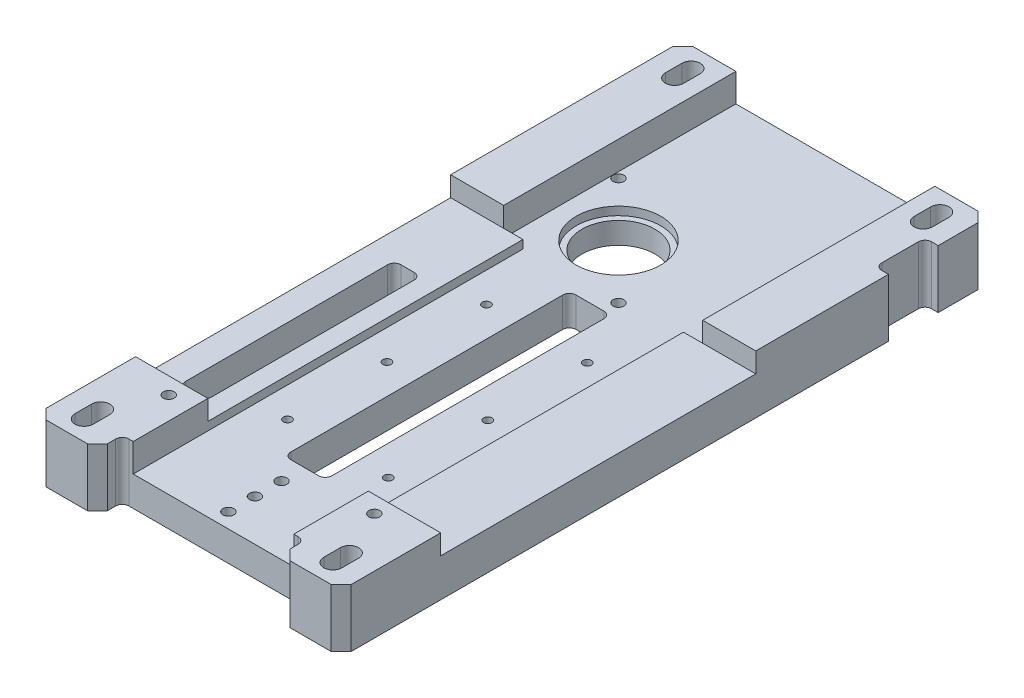
from build123d import *

# Parameters (mm, degrees)
SKETCH1_W               = 92
SKETCH1_H               = 230
BOSS_EXTRUDE1_DEPTH     = 17.5
SKETCH3_W               = 92
SKETCH3_H               = 20
CUT_EXTRUDE2_DEPTH      = 57
SKETCH7_W               = 92
SKETCH7_H               = 35
CUT_EXTRUDE5_DEPTH      = 70
SKETCH6_W               = 48.4
SKETCH6_H               = 175
CUT_EXTRUDE4_DEPTH      = 8.5
M3_TAPPED_HOLE1_D       = 2.5
SKETCH4_W               = 12.4
SKETCH4_H               = 86
CUT_EXTRUDE3_DEPTH      = 29
CHAMFER1_SIZE           = 3
FILLET1_R               = 2
SKETCH2_R               = 11
CUT_EXTRUDE1_DEPTH      = 10
BOSS_EXTRUDE2_DEPTH     = 20
CUT_EXTRUDE9_DEPTH      = 144.69150984
CHAMFER2_SIZE           = 3
SKETCH22_W              = 8
SKETCH22_H              = 65
CUT_EXTRUDE10_DEPTH     = 144.69150984
FILLET2_R               = 2
SKETCH12_R              = 12.75
CUT_EXTRUDE7_DEPTH      = 2.5
SKETCH23_W              = 92
SKETCH23_H              = 95
CUT_EXTRUDE11_DEPTH     = 6
M2_5_TAPPED_HOLE1_D     = 2.05
M2_5_TAPPED_HOLE1_DEPTH = 6.35
M2_5_TAPPED_HOLE1_TIP   = 0.615882135
M4_TAPPED_HOLE4_D       = 3.3
M4_TAPPED_HOLE4_DEPTH   = 10.1
M4_TAPPED_HOLE4_TIP     = 0.991420021
SKETCH16_R              = 1
CUT_EXTRUDE8_DEPTH      = 10
SKETCH30_W              = 4
SKETCH30_H              = 15
CUT_EXTRUDE12_DEPTH     = 144.69150984
M4_TAPPED_HOLE2_D       = 3.3
FILLET3_R               = 2
LPATTERN1_COUNT         = 3
LPATTERN1_PITCH         = 8
SKETCH31_W              = 55
SKETCH31_H              = 15
CUT_EXTRUDE13_DEPTH     = 27
FILLET4_R               = 2
CHAMFER3_SIZE           = 3
CUT_EXTRUDE14_REACH     = 145.692
SKETCH32_W              = 5.8
SKETCH32_H              = 70
M3_TAPPED_HOLE2_D       = 2.5
M3_TAPPED_HOLE2_DEPTH   = 7.5
M3_TAPPED_HOLE2_TIP     = 0.751075774
M3_TAPPED_HOLE3_D       = 2.5
M3_TAPPED_HOLE3_DEPTH   = 7.5
M3_TAPPED_HOLE3_TIP     = 0.751075774


with BuildPart() as part:
    # Sketch1 → Boss-Extrude1 (new body)
    with BuildSketch(Plane(origin=(0, 0, 0), x_dir=(1, 0, 0), z_dir=(0, 1, 0))):
        Rectangle(SKETCH1_W, SKETCH1_H)
    extrude(amount=BOSS_EXTRUDE1_DEPTH)

    # Sketch3 → Cut-Extrude2 (cut)
    with BuildSketch(Plane.XZ):
        with Locations((0, -105)):
            Rectangle(SKETCH3_W, SKETCH3_H)
    extrude(amount=-CUT_EXTRUDE2_DEPTH, mode=Mode.SUBTRACT)

    # Sketch7 → Cut-Extrude5 (cut)
    with BuildSketch(Plane.XZ):
        with Locations((0, -77.5)):
            Rectangle(SKETCH7_W, SKETCH7_H)
    extrude(amount=-CUT_EXTRUDE5_DEPTH, mode=Mode.SUBTRACT)

    # Sketch6 → Cut-Extrude4 (cut)
    with BuildSketch(Plane(origin=(0, 17.5, 0), x_dir=(1, 0, 0), z_dir=(0, 1, 0))):
        with Locations((0, -27.5)):
            Rectangle(SKETCH6_W, SKETCH6_H)
    extrude(amount=-CUT_EXTRUDE4_DEPTH, mode=Mode.SUBTRACT)

    # M3 Tapped Hole1 (through all)
    with Locations(Plane(origin=(0, 9, 0), x_dir=(1, 0, 0), z_dir=(0, 1, 0))):
        with Locations((15.2, -90), (-15.2, -90), (-15.2, -60), (15.2, -60), (15.2, -30), (-15.2, -30)):
            Hole(M3_TAPPED_HOLE1_D / 2)

    # Sketch4 → Cut-Extrude3 (cut)
    with BuildSketch(Plane.XZ):
        with Locations((0, 57)):
            Rectangle(SKETCH4_W, SKETCH4_H)
    extrude(amount=-CUT_EXTRUDE3_DEPTH, mode=Mode.SUBTRACT)

    # Chamfer1
    chamfer1_edges = [part.edges().sort_by_distance(p)[0] for p in [
        (46, 8.75, -60),
        (-46, 8.75, -60),
    ]]
    chamfer(chamfer1_edges, length=CHAMFER1_SIZE)

    # Fillet1
    fillet1_edges = [part.edges().sort_by_distance(p)[0] for p in [
        (6.2, 4.5, 100),
        (6.2, 4.5, 14),
        (-6.2, 4.5, 14),
        (-6.2, 4.5, 100),
    ]]
    fillet(fillet1_edges, radius=FILLET1_R)

    # Sketch2 → Cut-Extrude1 (cut)
    with BuildSketch(Plane.XZ):
        with Locations(Location((-12, -6.6, 0), (0, 0, 270))):
            Circle(SKETCH2_R)
    extrude(amount=-CUT_EXTRUDE1_DEPTH, mode=Mode.SUBTRACT)

    # Sketch20 → Boss-Extrude2 (add)
    with BuildSketch(Plane.XY.offset(115)):
        Polygon((-46, 17.5), (-24.2, 17.5), (-24.2, 9), (24.2, 9), (24.2, 17.5), (46, 17.5), (46, 0), (-46, 0), align=None)
    extrude(amount=BOSS_EXTRUDE2_DEPTH)

    # Sketch21 → Cut-Extrude9 (cut, through all)
    with BuildSketch(Plane.XZ):
        with BuildLine():
            Line((-34.75, 129), (-34.75, 124))
            ThreePointArc((-34.75, 124), (-37.5, 121.25), (-40.25, 124))
            Line((-40.25, 124), (-40.25, 129))
            ThreePointArc((-40.25, 129), (-37.5, 131.75), (-34.75, 129))
        make_face()
        with BuildLine():
            Line((34.75, 129), (34.75, 124))
            ThreePointArc((34.75, 124), (37.5, 121.25), (40.25, 124))
            Line((40.25, 124), (40.25, 129))
            ThreePointArc((40.25, 129), (37.5, 131.75), (34.75, 129))
        make_face()
        with BuildLine():
            Line((34.75, -54), (34.75, -49))
            ThreePointArc((34.75, -49), (37.5, -46.25), (40.25, -49))
            Line((40.25, -49), (40.25, -54))
            ThreePointArc((40.25, -54), (37.5, -56.75), (34.75, -54))
        make_face()
        with BuildLine():
            Line((-34.75, -54), (-34.75, -49))
            ThreePointArc((-34.75, -49), (-37.5, -46.25), (-40.25, -49))
            Line((-40.25, -49), (-40.25, -54))
            ThreePointArc((-40.25, -54), (-37.5, -56.75), (-34.75, -54))
        make_face()
    extrude(amount=-CUT_EXTRUDE9_DEPTH, mode=Mode.SUBTRACT)

    # Chamfer2
    chamfer2_edges = [part.edges().sort_by_distance(p)[0] for p in [
        (-46, 8.75, 135),
        (46, 8.75, 135),
    ]]
    chamfer(chamfer2_edges, length=CHAMFER2_SIZE)

    # Sketch22 → Cut-Extrude10 (cut, through all)
    with BuildSketch(Plane.XZ):
        with Locations((-34, 67.5)):
            Rectangle(SKETCH22_W, SKETCH22_H)
    extrude(amount=-CUT_EXTRUDE10_DEPTH, mode=Mode.SUBTRACT)

    # Fillet2
    fillet2_edges = [part.edges().sort_by_distance(p)[0] for p in [
        (-38, 8.75, 35),
        (-38, 8.75, 100),
        (-30, 8.75, 100),
        (-30, 8.75, 35),
    ]]
    fillet(fillet2_edges, radius=FILLET2_R)

    # Sketch12 → Cut-Extrude7 (cut)
    with BuildSketch(Plane(origin=(0, 9, 0), x_dir=(1, 0, 0), z_dir=(0, 1, 0))):
        with Locations(Location((-12, 6.6, 0), (0, 0, 270))):
            Circle(SKETCH12_R)
    extrude(amount=-CUT_EXTRUDE7_DEPTH, mode=Mode.SUBTRACT)

    # Sketch23 → Cut-Extrude11 (cut)
    with BuildSketch(Plane(origin=(0, 17.5, 0), x_dir=(1, 0, 0), z_dir=(0, 1, 0))):
        with Locations((0, -57.5)):
            Rectangle(SKETCH23_W, SKETCH23_H)
    extrude(amount=-CUT_EXTRUDE11_DEPTH, mode=Mode.SUBTRACT)

    # M2.5 Tapped Hole1
    with Locations(Plane(origin=(-10.2, 0, 83.891528236), x_dir=(0, 0, -1), z_dir=(0, -1, 0))):
        with Locations((0, 0), (13, 0)):
            Hole(M2_5_TAPPED_HOLE1_D / 2, depth=M2_5_TAPPED_HOLE1_DEPTH)
            with Locations((0, 0, -(M2_5_TAPPED_HOLE1_DEPTH + M2_5_TAPPED_HOLE1_TIP / 2))):  # 118° drill point
                Cone(0, M2_5_TAPPED_HOLE1_D / 2, M2_5_TAPPED_HOLE1_TIP, mode=Mode.SUBTRACT)

    # Sketch26 → M4 Tapped Hole3 (revolve, cut)
    with BuildSketch(Plane(origin=(0, 0, 107), x_dir=(0, 0, -1), z_dir=(1, 0, 0))):
        Polygon((0, 0), (0, 11.091420021), (1.65, 10.1), (1.65, 0), align=None)
    m4_tapped_hole3 = revolve(axis=Axis((0, -6.35, 107), (0, 1, 0)), mode=Mode.SUBTRACT)

    # M4 Tapped Hole4
    with Locations(Plane(origin=(0, 17.5, 0), x_dir=(1, 0, 0), z_dir=(0, 1, 0))):
        with Locations((31, -110), (-31, -110)):
            Hole(M4_TAPPED_HOLE4_D / 2, depth=M4_TAPPED_HOLE4_DEPTH)
            with Locations((0, 0, -(M4_TAPPED_HOLE4_DEPTH + M4_TAPPED_HOLE4_TIP / 2))):  # 118° drill point
                Cone(0, M4_TAPPED_HOLE4_D / 2, M4_TAPPED_HOLE4_TIP, mode=Mode.SUBTRACT)

    # Sketch16 → Cut-Extrude8 (cut)
    with BuildSketch(Plane.XZ):
        with Locations(Location((4.263455967, 9.663455967, 0), (0, 0, 270))):
            Circle(SKETCH16_R)
        with Locations(Location((-28.263455967, -22.863455967, 0), (0, 0, 270))):
            Circle(SKETCH16_R)
    extrude(amount=-CUT_EXTRUDE8_DEPTH, mode=Mode.SUBTRACT)

    # Sketch30 → Cut-Extrude12 (cut, through all)
    with BuildSketch(Plane.XZ):
        with Locations((44, -37.5)):
            Rectangle(SKETCH30_W, SKETCH30_H)
    extrude(amount=-CUT_EXTRUDE12_DEPTH, mode=Mode.SUBTRACT)

    # M4 Tapped Hole2 (through all)
    with Locations(Plane(origin=(-28.263455967, 0, -22.863455967), x_dir=(0, 0, -1), z_dir=(0, -1, 0))):
        with Locations((0, 0), (-32.526911934, 32.526911934)):
            Hole(M4_TAPPED_HOLE2_D / 2)

    # Fillet3
    fillet3_edges = [part.edges().sort_by_distance(p)[0] for p in [
        (42, 8.75, -45),
        (42, 8.75, -30),
    ]]
    fillet(fillet3_edges, radius=FILLET3_R)

    # LPattern1: M4 Tapped Hole3 ×3
    with Locations(*[(0, 0, i * LPATTERN1_PITCH) for i in range(1, LPATTERN1_COUNT)]):
        add(m4_tapped_hole3, mode=Mode.SUBTRACT)

    # Sketch31 → Cut-Extrude13 (cut)
    with BuildSketch(Plane.XZ):
        with Locations((0, 135)):
            Rectangle(SKETCH31_W, SKETCH31_H)
    extrude(amount=-CUT_EXTRUDE13_DEPTH, mode=Mode.SUBTRACT)

    # Fillet4
    fillet4_edges = [part.edges().sort_by_distance(p)[0] for p in [
        (27.5, 8.75, 127.5),
        (-27.5, 8.75, 127.5),
    ]]
    fillet(fillet4_edges, radius=FILLET4_R)

    # Chamfer3
    chamfer3_edges = [part.edges().sort_by_distance(p)[0] for p in [
        (-27.5, 8.75, 135),
        (27.5, 8.75, 135),
    ]]
    chamfer(chamfer3_edges, length=CHAMFER3_SIZE)

    # Cut-Extrude14: up to this face of the body (flat: up to its plane)
    cut_extrude14_end = Plane(part.part.faces().sort_by_distance((-0.202555348, 9, -15.347138665))[0])
    # Sketch32 → Cut-Extrude14 (cut, up to the picked face)
    with BuildSketch(Plane(origin=(0, 17.5, 0), x_dir=(1, 0, 0), z_dir=(0, 1, 0)), mode=Mode.PRIVATE) as cut_extrude14_sk1:
        with Locations((-27.1, 25)):
            Rectangle(SKETCH32_W, SKETCH32_H)
    cut_extrude14_tool1 = split(extrude(cut_extrude14_sk1.sketch, amount=-CUT_EXTRUDE14_REACH, mode=Mode.PRIVATE), bisect_by=cut_extrude14_end, keep=Keep.BOTH, mode=Mode.PRIVATE)
    # Sketch32 → Cut-Extrude14 (cut, up to the picked face)
    with BuildSketch(Plane(origin=(0, 17.5, 0), x_dir=(1, 0, 0), z_dir=(0, 1, 0)), mode=Mode.PRIVATE) as cut_extrude14_sk2:
        with Locations((27.1, 25)):
            Rectangle(SKETCH32_W, SKETCH32_H)
    cut_extrude14_tool2 = split(extrude(cut_extrude14_sk2.sketch, amount=-CUT_EXTRUDE14_REACH, mode=Mode.PRIVATE), bisect_by=cut_extrude14_end, keep=Keep.BOTH, mode=Mode.PRIVATE)
    add(cut_extrude14_tool1.solids().sort_by(Axis((-27.1, 17.5, -25), (0, -1, 0)))[0], mode=Mode.SUBTRACT)
    add(cut_extrude14_tool2.solids().sort_by(Axis((27.1, 17.5, -25), (0, -1, 0)))[0], mode=Mode.SUBTRACT)

    # M3 Tapped Hole2
    with Locations(Plane(origin=(0, 0, 0), x_dir=(-1, 0, 0), z_dir=(0, -1, 0))):
        with Locations((41, -22)):
            Hole(M3_TAPPED_HOLE2_D / 2, depth=M3_TAPPED_HOLE2_DEPTH)
            with Locations((0, 0, -(M3_TAPPED_HOLE2_DEPTH + M3_TAPPED_HOLE2_TIP / 2))):  # 118° drill point
                Cone(0, M3_TAPPED_HOLE2_D / 2, M3_TAPPED_HOLE2_TIP, mode=Mode.SUBTRACT)

    # M3 Tapped Hole3
    with Locations(Plane(origin=(0, 0, 0), x_dir=(-1, 0, 0), z_dir=(0, -1, 0))):
        with Locations((24, -113)):
            Hole(M3_TAPPED_HOLE3_D / 2, depth=M3_TAPPED_HOLE3_DEPTH)
            with Locations((0, 0, -(M3_TAPPED_HOLE3_DEPTH + M3_TAPPED_HOLE3_TIP / 2))):  # 118° drill point
                Cone(0, M3_TAPPED_HOLE3_D / 2, M3_TAPPED_HOLE3_TIP, mode=Mode.SUBTRACT)


solid = part.part
